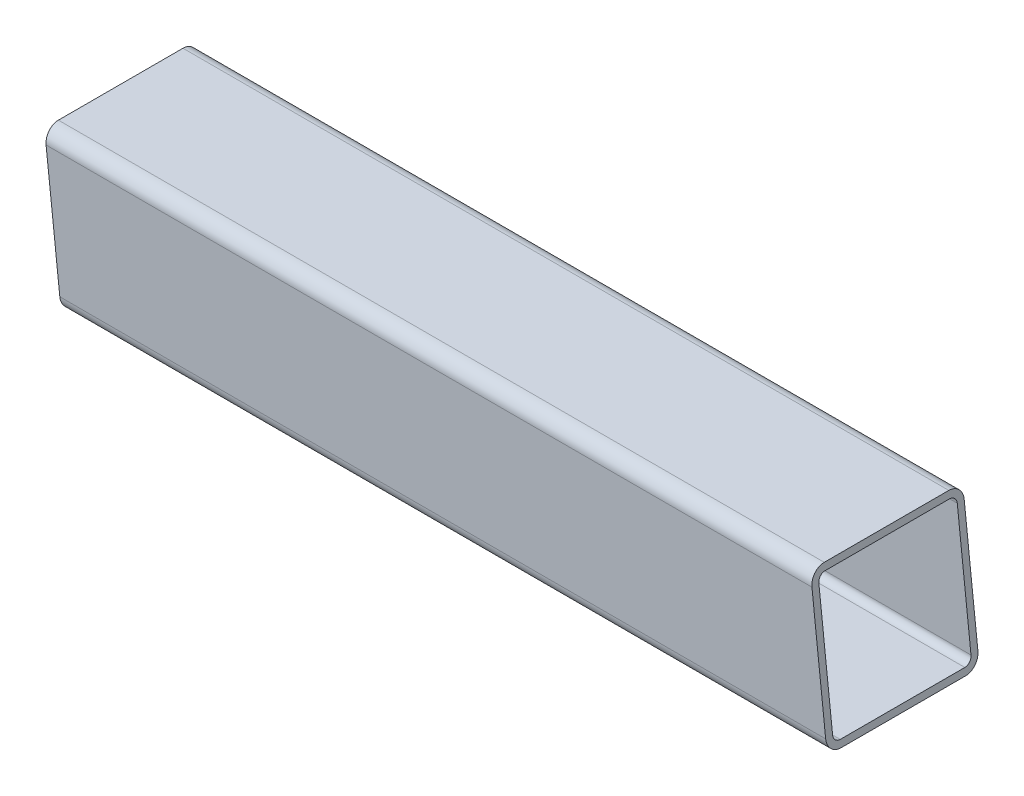
SolidWorks part; units mm, degrees
material "普通碳钢"
ref_plane "前视基准面" through (0, 0, 0) normal (0, 0, 1) x (1, 0, 0)
ref_plane "上视基准面" through (0, 0, 0) normal (0, 1, 0) x (1, 0, 0)
ref_plane "右视基准面" through (0, 0, 0) normal (1, 0, 0) x (0, 0, -1)
sketch3d "3D草图1"
  line L0 (0, 0, 0) -> (600, 0, 0)
  dimension "D1" = 600
other "方形管 110 X 110 X 5(1)"
ref_plane "基准面1" through (0, 0, 0) normal (1, 0, 0) x (0, 0, -1)
sketch "Sketch1" plane through (0, 0, 0) normal (1, 0, 0) x (0, 0, -1)
  line L0 (-45, -50) -> (45, -50)
  line L1 (-50, -45) -> (-50, 45)
  line L2 (45, 50) -> (-45, 50)
  line L3 (50, 45) -> (50, -45)
  line L4 (-45, -55) -> (45, -55)
  line L5 (-55, -45) -> (-55, 45)
  line L6 (45, 55) -> (-45, 55)
  line L7 (55, 45) -> (55, -45)
  arc A0 (55, 45) -> (45, 55) centre (45, 45) ccw
  arc A1 (45, -55) -> (55, -45) centre (45, -45) ccw
  arc A2 (-55, -45) -> (-45, -55) centre (-45, -45) ccw
  arc A3 (-45, 55) -> (-55, 45) centre (-45, 45) ccw
  arc A4 (-45, 50) -> (-50, 45) centre (-45, 45) ccw
  arc A5 (50, 45) -> (45, 50) centre (45, 45) ccw
  arc A6 (45, -50) -> (50, -45) centre (45, -45) ccw
  arc A7 (-50, -45) -> (-45, -50) centre (-45, -45) ccw
  point P0 (-55, 0)
  point P1 (55, 0)
  point P2 (0, 55)
  point P3 (0, -55)
  point P4 (0, 0)
  point P5 (-55, -55)
  point P6 (55, -55)
  point P7 (55, 55)
  point P8 (-55, 55)
  point P33 (0, 0)
  dimension "D1" = 10
  dimension "Thickness" = 5
  dimension "V_leg" = 110
sketch "草图2" plane through (0, 0, 55) normal (0, 0, 1) x (1, 0, 0)
  line L0 (0, 148.5831) -> (22.456, -55)
  line L1 (600, -55) -> (0, -55) construction
  line L2 (22.456, -55) -> (0, -55)
  line L3 (0, -55) -> (0, 148.5831)
  line L4 (600, -274.468) -> (563.6584, 55)
  line L5 (600, 55) -> (0, 55) construction
  line L6 (563.6584, 55) -> (600, 55)
  line L7 (600, 55) -> (600, -274.468)
  line L8 (22.456, -55) -> (569.1403, 5.3014) construction
  line L9 (600, 45) -> (600, 55) construction
  dimension "D1" = 550
  dimension "D2" = 50
extrude "切除-拉伸1" cut sketch "草图2" against normal up to surface (110 mm away) up to face at (300, 0, -55)
